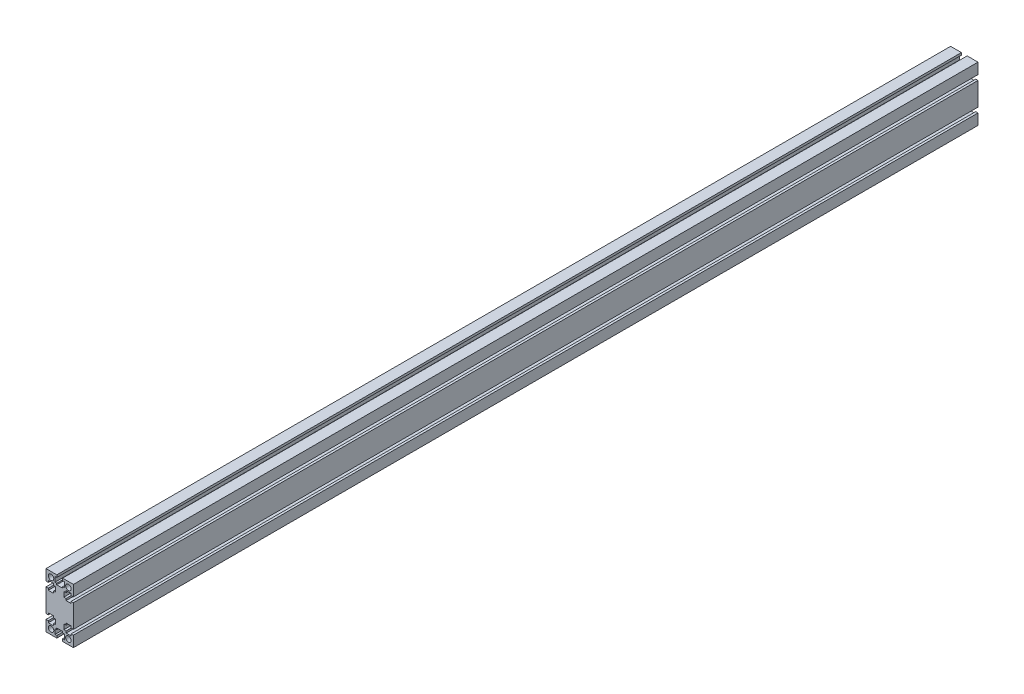
from build123d import *

# Parameters (mm, degrees)
SKETCH_1_R      = 3
EXTRUDE_1_DEPTH = 990


with BuildPart() as part:
    # 草图1 → 凸台-拉伸1 (new body)
    with BuildSketch(Plane.XY):
        Polygon((-27.495741056, 11.192504259), (-24.995741056, 11.192504259), (-24.995741056, 13.192504259), (-19.495741056, 13.192504259), (-19.495741056, 11.192504259), (-16.995741056, 11.192504259), (-16.995741056, 5.692504259), (-19.495741056, 5.692504259), (-19.495741056, 3.692504259), (-24.995741056, 3.692504259), (-24.995741056, 5.692504259), (-27.495741056, 5.692504259), (-27.495741056, -19.607495741), (-24.995741056, -19.607495741), (-24.995741056, -17.607495741), (-19.495741056, -17.607495741), (-19.495741056, -19.607495741), (-16.995741056, -19.607495741), (-16.995741056, -25.107495741), (-19.495741056, -25.107495741), (-19.495741056, -27.107495741), (-24.995741056, -27.107495741), (-24.995741056, -25.107495741), (-27.495741056, -25.107495741), (-27.495741056, -36.957495741), (-15.645741056, -36.957495741), (-15.645741056, -34.457495741), (-17.645741056, -34.457495741), (-17.645741056, -28.957495741), (-15.748076247, -28.957495741), (-15.748076247, -27.422563567), (-9.243405866, -27.422563567), (-9.243405866, -28.957495741), (-7.345741056, -28.957495741), (-7.345741056, -34.457495741), (-9.345741056, -34.457495741), (-9.345741056, -36.957495741), (2.504258944, -36.957495741), (2.504258944, -25.107495741), (0.004258944, -25.107495741), (0.004258944, -27.107495741), (-5.495741056, -27.107495741), (-5.495741056, -25.107495741), (-7.995741056, -25.107495741), (-7.995741056, -19.607495741), (-5.495741056, -19.607495741), (-5.495741056, -17.607495741), (0.004258944, -17.607495741), (0.004258944, -19.607495741), (2.504258944, -19.607495741), (2.504258944, 5.692504259), (0.004258944, 5.692504259), (0.004258944, 3.692504259), (-5.495741056, 3.692504259), (-5.495741056, 5.692504259), (-7.995741056, 5.692504259), (-7.995741056, 11.192504259), (-5.495741056, 11.192504259), (-5.495741056, 13.192504259), (0.004258944, 13.192504259), (0.004258944, 11.192504259), (2.504258944, 11.192504259), (2.504258944, 23.042504259), (-9.345741056, 23.042504259), (-9.345741056, 20.542504259), (-7.345741056, 20.542504259), (-7.345741056, 15.042504259), (-9.243405866, 15.042504259), (-9.243405866, 13.507572085), (-15.748076247, 13.507572085), (-15.748076247, 15.042504259), (-17.645741056, 15.042504259), (-17.645741056, 20.542504259), (-15.645741056, 20.542504259), (-15.645741056, 23.042504259), (-27.495741056, 23.042504259), align=None)
        with Locations((-21.995741056, 17.542504259)):
            Circle(SKETCH_1_R, mode=Mode.SUBTRACT)
        with Locations(Location((-2.995741056, 17.542504259, 0), (0, 0, 180))):
            Circle(SKETCH_1_R, mode=Mode.SUBTRACT)
        with Locations((-2.995741056, -31.457495741)):
            Circle(SKETCH_1_R, mode=Mode.SUBTRACT)
        with Locations(Location((-21.995741056, -31.457495741, 0), (0, 0, 180))):
            Circle(SKETCH_1_R, mode=Mode.SUBTRACT)
    extrude(amount=EXTRUDE_1_DEPTH)


solid = part.part
